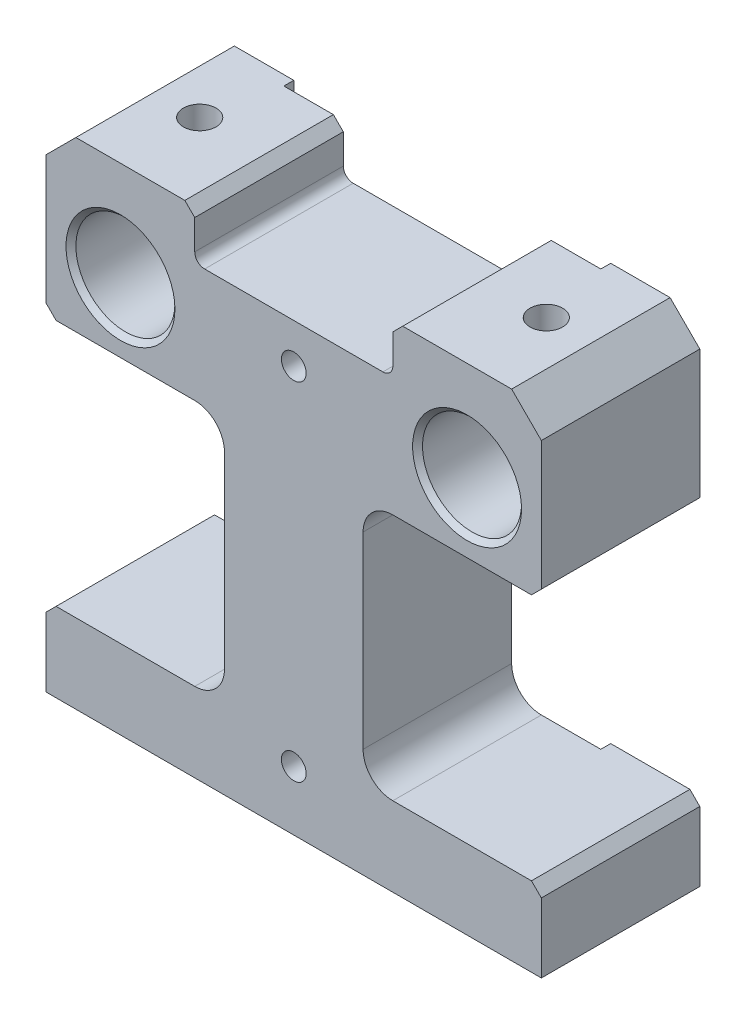
from build123d import *

# Parameters (mm, degrees)
BOSS_EXTRUDE1_DEPTH    = 8
SKETCH6_R              = 5
SKETCH6_W              = 18
SKETCH6_H              = 25
CUT_EXTRUDE1_DEPTH     = 39.807215824
M4_TAPPED_HOLE1_REACH  = 58.471
M4_TAPPED_HOLE1_BORE_R = 1.65
M3_TAPPED_HOLE1_D      = 2.5
SKETCH13_W             = 32
SKETCH13_H             = 50
CUT_EXTRUDE2_DEPTH     = 1
SKETCH14_W             = 20
SKETCH14_H             = 5
CUT_EXTRUDE3_DEPTH     = 39.80721593
CHAMFER1_SIZE          = 3
FILLET1_R              = 3
CHAMFER3_SIZE          = 1
CHAMFER4_SIZE          = 0.5
FILLET2_R              = 1


with BuildPart() as part:
    # Sketch1 → Boss-Extrude1 (new, symmetric)
    with BuildSketch(Plane.XY):
        Polygon((-25, -10), (-25, -25), (25, -25), (25, -10), (25, 25), (-25, 25), align=None)
    extrude(amount=BOSS_EXTRUDE1_DEPTH, both=True)

    # Sketch6 → Cut-Extrude1 (cut, through all)
    with BuildSketch(Plane.XY.offset(8)):
        with Locations((-17.5, 15)):
            Circle(SKETCH6_R)
        with Locations((17.5, 15)):
            Circle(SKETCH6_R)
        with Locations((16, -4.5)):
            Rectangle(SKETCH6_W, SKETCH6_H)
        with Locations((-16, -4.5)):
            Rectangle(SKETCH6_W, SKETCH6_H)
    extrude(amount=-CUT_EXTRUDE1_DEPTH, mode=Mode.SUBTRACT)

    # M4 Tapped Hole1 bore → M4 Tapped Hole1 (cut, up to next)
    with BuildSketch(Plane(origin=(0, 25, 0), x_dir=(1, 0, 0), z_dir=(0, 1, 0)), mode=Mode.PRIVATE) as m4_tapped_hole1_sk1:
        with Locations((-17.5, 0)):
            Circle(M4_TAPPED_HOLE1_BORE_R)
    m4_tapped_hole1_tool1 = extrude(m4_tapped_hole1_sk1.sketch, amount=-M4_TAPPED_HOLE1_REACH, mode=Mode.PRIVATE) & part.part
    # M4 Tapped Hole1 bore → M4 Tapped Hole1 (cut, up to next)
    with BuildSketch(Plane(origin=(0, 25, 0), x_dir=(1, 0, 0), z_dir=(0, 1, 0)), mode=Mode.PRIVATE) as m4_tapped_hole1_sk2:
        with Locations((17.5, 0)):
            Circle(M4_TAPPED_HOLE1_BORE_R)
    m4_tapped_hole1_tool2 = extrude(m4_tapped_hole1_sk2.sketch, amount=-M4_TAPPED_HOLE1_REACH, mode=Mode.PRIVATE) & part.part
    add(m4_tapped_hole1_tool1.solids().sort_by_distance((-17.5, 25, 0))[0], mode=Mode.SUBTRACT)
    add(m4_tapped_hole1_tool2.solids().sort_by_distance((17.5, 25, 0))[0], mode=Mode.SUBTRACT)

    # M3 Tapped Hole1 (through all)
    with Locations(Plane.XY.offset(8)):
        with Locations((0, -19), (0, 16)):
            Hole(M3_TAPPED_HOLE1_D / 2)

    # Sketch13 → Cut-Extrude2 (cut)
    with BuildSketch(Plane.XY.offset(-8)):
        Rectangle(SKETCH13_W, SKETCH13_H)
    extrude(amount=CUT_EXTRUDE2_DEPTH, mode=Mode.SUBTRACT)

    # Sketch14 → Cut-Extrude3 (cut, through all)
    with BuildSketch(Plane.XY.offset(8)):
        with Locations((0, 22.5)):
            Rectangle(SKETCH14_W, SKETCH14_H)
    extrude(amount=-CUT_EXTRUDE3_DEPTH, mode=Mode.SUBTRACT)

    # Chamfer1
    chamfer1_edges = [part.edges().sort_by_distance(p)[0] for p in [
        (-25, 25, 0),
        (25, 25, 0),
    ]]
    chamfer(chamfer1_edges, length=CHAMFER1_SIZE)

    # Fillet1
    fillet1_edges = [part.edges().sort_by_distance(p)[0] for p in [
        (-7, -17, 0.5),
        (-7, 8, 0.5),
        (7, -17, 0.5),
        (7, 8, 0.5),
    ]]
    fillet(fillet1_edges, radius=FILLET1_R)

    # Chamfer3
    chamfer3_edges = [part.edges().sort_by_distance(p)[0] for p in [
        (-10, 25, 0.5),
        (10, 25, 0.5),
        (25, 8, 0),
        (25, -17, 0),
        (-25, -17, 0),
        (-25, 8, 0),
    ]]
    chamfer(chamfer3_edges, length=CHAMFER3_SIZE)

    # Chamfer4
    chamfer4_edges = [part.edges().sort_by_distance(p)[0] for p in [
        (-22.5, 15, -8),
        (-22.5, 15, 8),
        (12.5, 15, 8),
        (20.458039892, 19.031128874, -8),
    ]]
    chamfer(chamfer4_edges, length=CHAMFER4_SIZE)

    # Fillet2
    fillet2_edges = [part.edges().sort_by_distance(p)[0] for p in [
        (-10, 20, 0.5),
        (10, 20, 0.5),
    ]]
    fillet(fillet2_edges, radius=FILLET2_R)


solid = part.part
